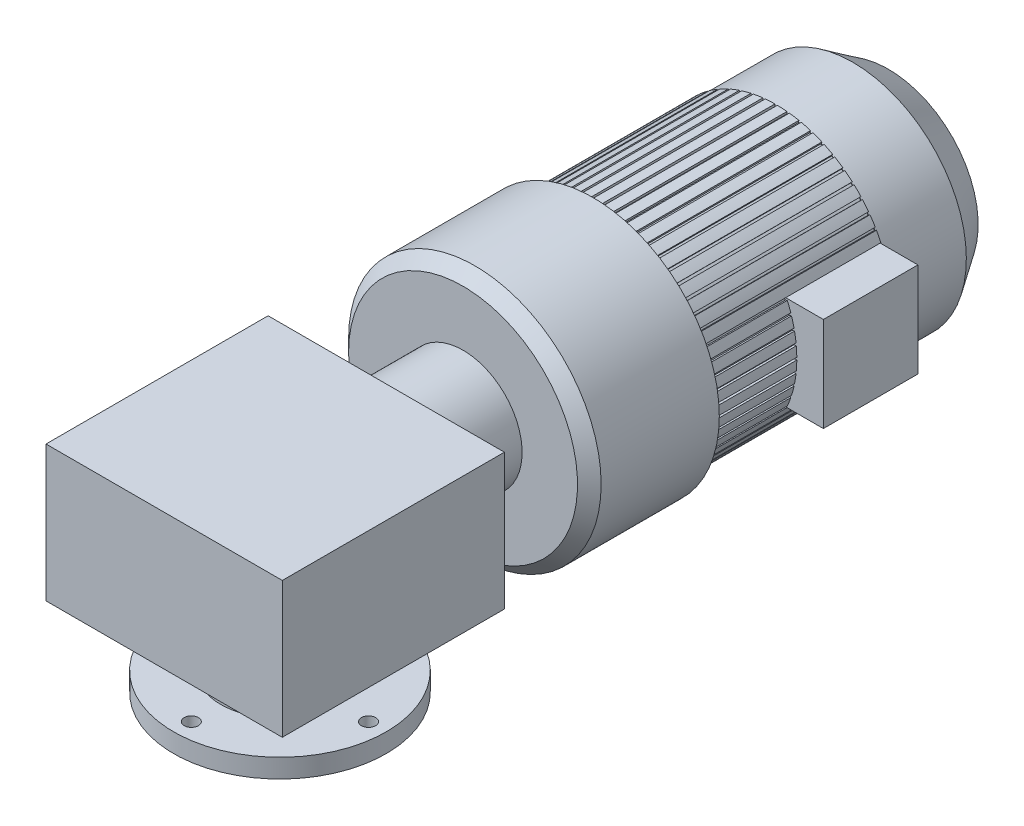
from build123d import *

# Parameters (mm, degrees)
SKETCH1_R            = 16
BOSS_EXTRUDE1_DEPTH  = 55
SKETCH2_R            = 22.5
BOSS_EXTRUDE2_DEPTH  = 5
SKETCH3_R            = 25
BOSS_EXTRUDE3_DEPTH  = 5
SKETCH4_R            = 50
BOSS_EXTRUDE4_DEPTH  = 65
SKETCH5_R            = 106.9
BOSS_EXTRUDE5_DEPTH  = 110
SKETCH6_R            = 97.5
BOSS_EXTRUDE6_DEPTH  = 155
SKETCH7_W            = 2
SKETCH7_H            = 4
CUT_EXTRUDE1_DEPTH   = 155
CIRPATTERN1_COUNT    = 60
SKETCH8_R            = 96
BOSS_EXTRUDE7_DEPTH  = 95
CHAMFER1_SIZE        = 30
CHAMFER1_SIZE2       = 20
SKETCH13_W           = 80
SKETCH13_H           = 80
BOSS_EXTRUDE8_DEPTH  = 120
SKETCH14_W           = 200
SKETCH14_H           = 115
BOSS_EXTRUDE9_DEPTH  = 188
SKETCH15_R           = 50
BOSS_EXTRUDE10_DEPTH = 50
SKETCH16_R           = 90
SKETCH16_R_2         = 6
BOSS_EXTRUDE11_DEPTH = 16
CHAMFER2_SIZE        = 10


with BuildPart() as part:
    # Sketch1 → Boss-Extrude1 (new body)
    with BuildSketch(Plane.XY):
        Circle(SKETCH1_R)
    extrude(amount=BOSS_EXTRUDE1_DEPTH)

    # Sketch2 → Boss-Extrude2 (add)
    with BuildSketch(Plane(origin=(0, 0, 0), x_dir=(-1, 0, 0), z_dir=(0, 0, -1))):
        Circle(SKETCH2_R)
    extrude(amount=BOSS_EXTRUDE2_DEPTH)

    # Sketch3 → Boss-Extrude3 (add)
    with BuildSketch(Plane(origin=(0, 0, -5), x_dir=(-1, 0, 0), z_dir=(0, 0, -1))):
        Circle(SKETCH3_R)
    extrude(amount=BOSS_EXTRUDE3_DEPTH)

    # Sketch4 → Boss-Extrude4 (add)
    with BuildSketch(Plane(origin=(0, 0, -10), x_dir=(-1, 0, 0), z_dir=(0, 0, -1))):
        with Locations(Location((0, -30.4, 0), (0, 0, 112.960160848))):
            Circle(SKETCH4_R)
    extrude(amount=BOSS_EXTRUDE4_DEPTH)

    # Sketch5 → Boss-Extrude5 (add)
    with BuildSketch(Plane(origin=(0, 0, -75), x_dir=(-1, 0, 0), z_dir=(0, 0, -1))):
        with Locations((0, -30.4)):
            Circle(SKETCH5_R)
    extrude(amount=BOSS_EXTRUDE5_DEPTH)

    # Sketch6 → Boss-Extrude6 (add)
    with BuildSketch(Plane(origin=(0, 0, -185), x_dir=(-1, 0, 0), z_dir=(0, 0, -1))):
        with Locations((0, -30.4)):
            Circle(SKETCH6_R)
    extrude(amount=BOSS_EXTRUDE6_DEPTH)

    # Sketch7 → Cut-Extrude1 (cut)
    with BuildSketch(Plane(origin=(0, 0, -340), x_dir=(-1, 0, 0), z_dir=(0, 0, -1))):
        with Locations((0, 67.1)):
            Rectangle(SKETCH7_W, SKETCH7_H)
    cut_extrude1 = extrude(amount=-CUT_EXTRUDE1_DEPTH, mode=Mode.SUBTRACT)

    # CirPattern1: Cut-Extrude1 ×60 about axis
    cirpattern1_axis = Axis((0, -30.4, 0), (0, 0, 1))
    for i in range(1, CIRPATTERN1_COUNT):
        add(cut_extrude1.rotate(cirpattern1_axis, i * 360 / CIRPATTERN1_COUNT), mode=Mode.SUBTRACT)

    # Sketch8 → Boss-Extrude7 (add)
    with BuildSketch(Plane(origin=(0, 0, -340), x_dir=(-1, 0, 0), z_dir=(0, 0, -1))):
        with Locations(Location((0, -30.4, 0), (0, 0, 180.596841831))):
            Circle(SKETCH8_R)
    extrude(amount=BOSS_EXTRUDE7_DEPTH)

    # Chamfer1
    chamfer1_edges = [part.edges().sort_by_distance(p)[0] for p in [
        (-95.994791525, -29.399999999, -435),
    ]]
    chamfer1_side = [part.faces().sort_by_distance(p)[0] for p in [
        (-95.994791525, -29.399999999, -387.5),
    ]]
    chamfer(chamfer1_edges, length=CHAMFER1_SIZE, length2=CHAMFER1_SIZE2, reference=chamfer1_side[0])

    # Sketch13 → Boss-Extrude8 (add)
    with BuildSketch(Plane(origin=(0, 0, 0), x_dir=(0, 0, -1), z_dir=(1, 0, 0))):
        with Locations((300, -30.4)):
            Rectangle(SKETCH13_W, SKETCH13_H)
    extrude(amount=BOSS_EXTRUDE8_DEPTH)

    # Sketch14 → Boss-Extrude9 (add)
    with BuildSketch(Plane.XY.offset(-10)):
        with Locations((0, -30.19836827)):
            Rectangle(SKETCH14_W, SKETCH14_H)
    extrude(amount=BOSS_EXTRUDE9_DEPTH)

    # Sketch15 → Boss-Extrude10 (add)
    with BuildSketch(Plane(origin=(0, -87.69836827, 0), x_dir=(-1, 0, 0), z_dir=(0, -1, 0))):
        with Locations((0, -80)):
            Circle(SKETCH15_R)
    extrude(amount=BOSS_EXTRUDE10_DEPTH)

    # Sketch16 → Boss-Extrude11 (add)
    with BuildSketch(Plane(origin=(0, -137.69836827, 0), x_dir=(-1, 0, 0), z_dir=(0, -1, 0))):
        with Locations(Location((0, -80, 0), (0, 0, 90))):
            Circle(SKETCH16_R)
        with Locations(Location((0, -5, 0), (0, 0, 90))):
            Circle(SKETCH16_R_2, mode=Mode.SUBTRACT)
        with Locations(Location((-75, -80, 0), (0, 0, 90))):
            Circle(SKETCH16_R_2, mode=Mode.SUBTRACT)
        with Locations(Location((75, -80, 0), (0, 0, 90))):
            Circle(SKETCH16_R_2, mode=Mode.SUBTRACT)
        with Locations(Location((0, -155, 0), (0, 0, 90))):
            Circle(SKETCH16_R_2, mode=Mode.SUBTRACT)
    extrude(amount=BOSS_EXTRUDE11_DEPTH)

    # Chamfer2
    chamfer2_edges = [part.edges().sort_by_distance(p)[0] for p in [
        (106.9, -30.4, -75),
    ]]
    chamfer(chamfer2_edges, length=CHAMFER2_SIZE)


solid = part.part
